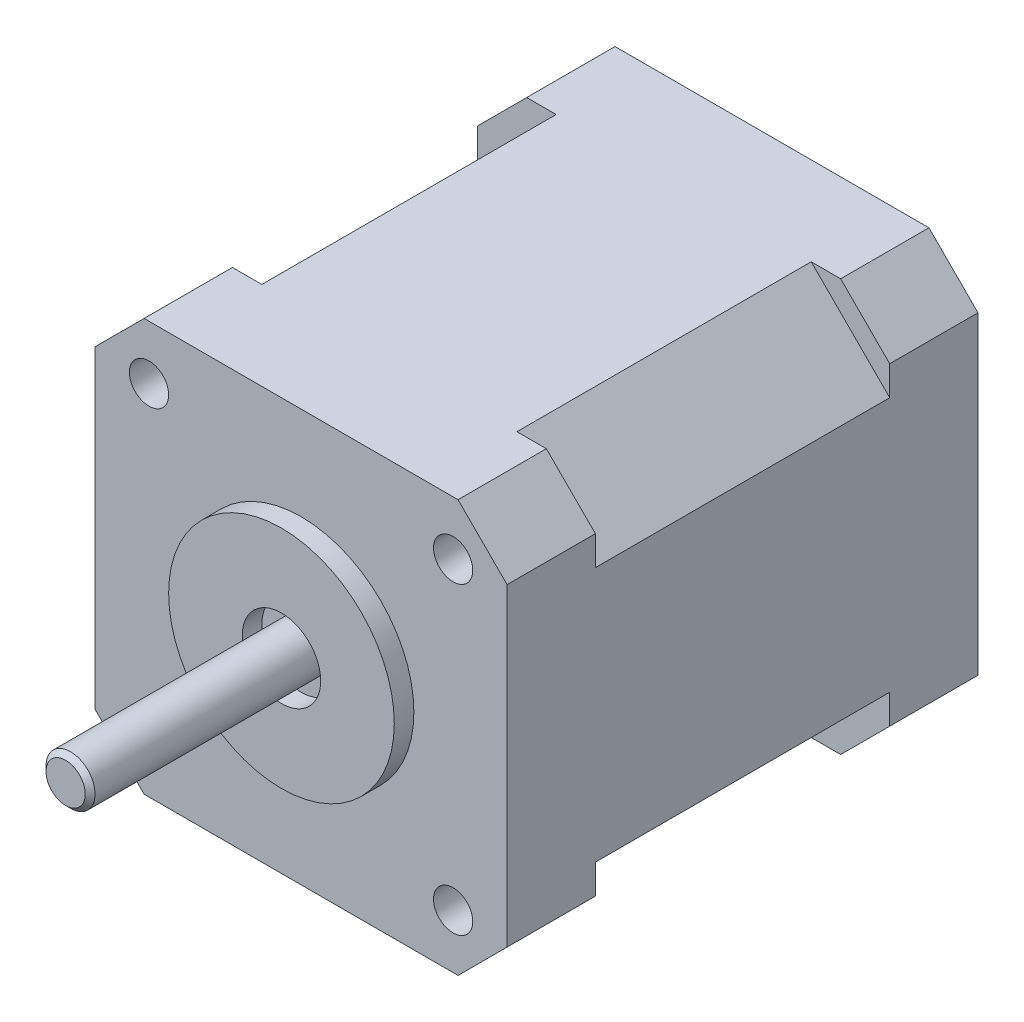
from build123d import *

# Parameters (mm, degrees)
SKETCH1_W           = 42
SKETCH1_H           = 42
BOSS_EXTRUDE1_DEPTH = 15
CHAMFER1_SIZE       = 8
BOSS_EXTRUDE2_DEPTH = 9
SKETCH4_R           = 11.5
BOSS_EXTRUDE3_DEPTH = 2
SKETCH5_R           = 2.5
BOSS_EXTRUDE4_DEPTH = 22
CUT_EXTRUDE1_START  = -2
SKETCH6_R           = 4
SKETCH6_R_2         = 2.5
CUT_EXTRUDE1_DEPTH  = 2
CHAMFER2_SIZE       = 0.5
SKETCH7_R           = 2
CUT_EXTRUDE2_DEPTH  = 57.444663167


with BuildPart() as part:
    # Sketch1 → Boss-Extrude1 (new, symmetric)
    with BuildSketch(Plane.XY):
        Rectangle(SKETCH1_W, SKETCH1_H)
    extrude(amount=BOSS_EXTRUDE1_DEPTH, both=True)

    # Chamfer1
    chamfer1_edges = [part.edges().sort_by_distance(p)[0] for p in [
        (-21, 21, 0),
        (21, 21, 0),
        (21, -21, 0),
        (-21, -21, 0),
    ]]
    chamfer(chamfer1_edges, length=CHAMFER1_SIZE)

    # Sketch3 → Boss-Extrude2 (add)
    with BuildSketch(Plane.XY.offset(15)):
        Polygon((16, -21), (-16, -21), (-21, -16), (-21, 16), (-16, 21), (16, 21), (21, 16), (21, -16), align=None)
    boss_extrude2 = extrude(amount=BOSS_EXTRUDE2_DEPTH)

    # Mirror1: Boss-Extrude2 across plane
    add(boss_extrude2.mirror(Plane.XY))

    # Sketch4 → Boss-Extrude3 (add)
    with BuildSketch(Plane.XY.offset(24)):
        with Locations(Location((0, 0, 0), (0, 0, 180))):
            Circle(SKETCH4_R)
    extrude(amount=BOSS_EXTRUDE3_DEPTH)

    # Sketch5 → Boss-Extrude4 (add)
    with BuildSketch(Plane.XY.offset(26)):
        Circle(SKETCH5_R)
    extrude(amount=BOSS_EXTRUDE4_DEPTH)

    # Sketch6 → Cut-Extrude1 (cut)
    with BuildSketch(Plane.XY.offset(26).offset(CUT_EXTRUDE1_START)):
        Circle(SKETCH6_R)
        Circle(SKETCH6_R_2, mode=Mode.SUBTRACT)
    extrude(amount=CUT_EXTRUDE1_DEPTH, mode=Mode.SUBTRACT)

    # Chamfer2
    chamfer2_edges = [part.edges().sort_by_distance(p)[0] for p in [
        (-2.5, 0, 48),
    ]]
    chamfer(chamfer2_edges, length=CHAMFER2_SIZE)

    # Sketch7 → Cut-Extrude2 (cut, through all)
    with BuildSketch(Plane.XY.offset(24)):
        with Locations((15.5, 15.5)):
            Circle(SKETCH7_R)
        with Locations((15.5, -15.5)):
            Circle(SKETCH7_R)
        with Locations((-15.5, -15.5)):
            Circle(SKETCH7_R)
        with Locations((-15.5, 15.5)):
            Circle(SKETCH7_R)
    extrude(amount=-CUT_EXTRUDE2_DEPTH, mode=Mode.SUBTRACT)


solid = part.part
